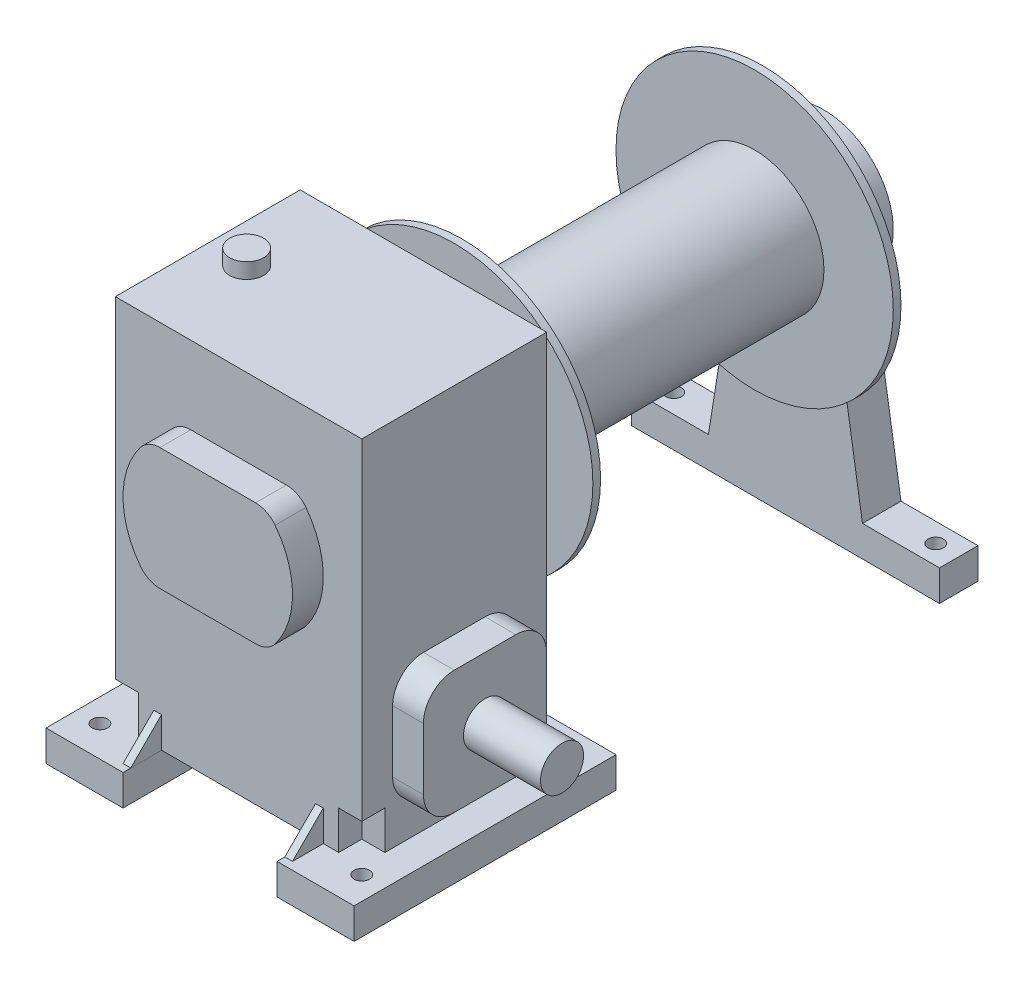
from build123d import *

# Parameters (mm, degrees)
EXTRUDE_1_DEPTH      = 20
EXTRUDE_1_DEPTH_BACK = 240
SKETCH_2_R           = 10
SKETCH_3_W           = 160
SKETCH_3_H           = 240
EXTRUDE_2_DEPTH      = 120
SKETCH_4_R           = 10
EXTRUDE_3_DEPTH      = 25
EXTRUDE_4_DEPTH      = 20
EXTRUDE_5_DEPTH      = 20
EXTRUDE_5_DEPTH_BACK = 180
SKETCH_7_W           = 80
SKETCH_7_H           = 80
FILLET_1_R           = 20
FILLET_2_R           = 16
SKETCH_8_R           = 14
EXTRUDE_6_DEPTH      = 50
SKETCH_10_W          = 50
SKETCH_10_H          = 20
EXTRUDE_7_DEPTH      = 85
EXTRUDE_7_2_DEPTH    = 85
EXTRUDE_8_DEPTH      = 5
SKETCH_12_R          = 5
CUT_EXTRUDE_1_DEPTH  = 20
SKETCH_13_W          = 15
SKETCH_13_H          = 15
CUT_EXTRUDE_2_DEPTH  = 25
SKETCH_14_R          = 11
EXTRUDE_9_DEPTH      = 10


with BuildPart() as part:
    # 草图1 → 旋转1 (revolve)
    with BuildSketch(Plane(origin=(0, 0, 0), x_dir=(0, 0, -1), z_dir=(1, 0, 0)), mode=Mode.PRIVATE) as revolve_1_sk:
        Polygon((-92.42282507, 0), (105.622076707, 0), (105.622076707, 90), (100.622076707, 90), (100.622076707, 45), (-89.377923293, 45), (-89.377923293, 90), (-94.377923293, 90), (-94.377923293, 0), align=None)
    revolve(revolve_1_sk.sketch.rotate(Axis((0, 0, 1000), (0, 0, -1)), 90), axis=Axis((0, 0, 1000), (0, 0, -1)))

    # 草图2 → 凸台-拉伸1 (add, two sides: drawn at the far end of the back side and taken through both)
    with BuildSketch(Plane.XY.offset(94.377923293).offset(-EXTRUDE_1_DEPTH_BACK)):
        Circle(SKETCH_2_R)
    extrude(amount=EXTRUDE_1_DEPTH + EXTRUDE_1_DEPTH_BACK)

    # 草图3 → 凸台-拉伸2 (add)
    with BuildSketch(Plane.XY.offset(114.377923293)):
        with Locations((0, -30)):
            Rectangle(SKETCH_3_W, SKETCH_3_H)
    extrude(amount=EXTRUDE_2_DEPTH)

    # 草图6 → 凸台-拉伸4 (add)
    with BuildSketch(Plane.XY.offset(234.377923293)):
        with BuildLine():
            Line((-38.147465423, 39.620334196), (38.147465423, 39.620334196))
            ThreePointArc((38.147465423, 39.620334196), (55, 0), (38.147465423, -39.620334196))
            Line((38.147465423, -39.620334196), (-38.147465423, -39.620334196))
            ThreePointArc((-38.147465423, -39.620334196), (-55, 0), (-38.147465423, 39.620334196))
        make_face()
    extrude(amount=EXTRUDE_4_DEPTH)

    # 草图7 → 凸台-拉伸5 (add, two sides: drawn at the far end of the back side and taken through both)
    with BuildSketch(Plane(origin=(80, 0, 0), x_dir=(0, 0, -1), z_dir=(1, 0, 0)).offset(-EXTRUDE_5_DEPTH_BACK)):
        with Locations((-174.377923293, -90)):
            Rectangle(SKETCH_7_W, SKETCH_7_H)
    extrude(amount=EXTRUDE_5_DEPTH + EXTRUDE_5_DEPTH_BACK)

    # 圆角1
    fillet_1_edges = [part.edges().sort_by_distance(p)[0] for p in [
        (90, -50, 134.377923293),
        (-90, -50, 134.377923293),
        (90, -130, 134.377923293),
        (-90, -130, 134.377923293),
        (90, -130, 214.377923293),
        (-90, -130, 214.377923293),
        (90, -50, 214.377923293),
        (-90, -50, 214.377923293),
    ]]
    fillet(fillet_1_edges, radius=FILLET_1_R)

    # 圆角2
    fillet_2_edges = [part.edges().sort_by_distance(p)[0] for p in [
        (-38.147465423, 39.620334196, 244.377923293),
        (-38.147465423, -39.620334196, 244.377923293),
        (38.147465423, -39.620334196, 244.377923293),
        (38.147465423, 39.620334196, 244.377923293),
    ]]
    fillet(fillet_2_edges, radius=FILLET_2_R)

    # 草图8 → 凸台-拉伸6 (add)
    with BuildSketch(Plane(origin=(100, 0, 0), x_dir=(0, 0, -1), z_dir=(1, 0, 0))):
        with Locations(Location((-174.377923293, -90, 0), (0, 0, 180))):
            Circle(SKETCH_8_R)
    extrude(amount=EXTRUDE_6_DEPTH)



with BuildPart() as body_2:
    # 草图4 → 凸台-拉伸3 (new body)
    with BuildSketch(Plane(origin=(0, 0, -145.622076707), x_dir=(-1, 0, 0), z_dir=(0, 0, -1))):
        with BuildLine():
            Line((-50, -150), (-100, -150))
            Line((-100, -150), (-100, -170))
            Line((-100, -170), (100, -170))
            Line((100, -170), (100, -150))
            Line((100, -150), (50, -150))
            Line((50, -150), (31.211895674, -32.416316392))
            ThreePointArc((31.211895674, -32.416316392), (41.40975311, -17.613413847), (45, 0))
            ThreePointArc((45, 0), (0, 45), (-45, 0))
            ThreePointArc((-45, 0), (-41.40975311, -17.613413847), (-31.211895674, -32.416316392))
            Line((-31.211895674, -32.416316392), (-50, -150))
        make_face()
        Circle(SKETCH_4_R, mode=Mode.SUBTRACT)
    extrude(amount=-EXTRUDE_3_DEPTH)


with BuildPart() as body_3:
    # 草图10 → 凸台-拉伸7 (new, symmetric)
    with BuildSketch(Plane.XY.offset(174.377923293)):
        with Locations((75, -160)):
            Rectangle(SKETCH_10_W, SKETCH_10_H)
    extrude(amount=EXTRUDE_7_DEPTH, both=True)


with BuildPart() as body_4:
    # 草图10 → Extrude 7 2 (new, symmetric)
    with BuildSketch(Plane.XY.offset(174.377923293)):
        with Locations((-75, -160)):
            Rectangle(SKETCH_10_W, SKETCH_10_H)
    extrude(amount=EXTRUDE_7_2_DEPTH, both=True)


with BuildPart() as part_1:
    add(part.part)

    add(body_3.part)  # 凸台-拉伸8 merges body 3
    # 草图11 → 凸台-拉伸8 (add)
    with BuildSketch(Plane.ZY.offset(-50)):
        Polygon((114.377923293, -130), (94.377923293, -150), (114.377923293, -150), align=None)
        Polygon((234.377923293, -130), (234.377923293, -150), (254.377923293, -150), align=None)
    extrude_8 = extrude(amount=-EXTRUDE_8_DEPTH)

    # 镜向1: 凸台-拉伸8 across plane
    add(extrude_8.mirror(Plane(origin=(0, 0, 0), x_dir=(0, 0, 1), z_dir=(1, 0, 0))))


with BuildPart() as cut_extrude_1_tool:
    # 草图12 → 切除-拉伸1 (new body)
    with BuildSketch(Plane.XZ.offset(170)):
        with Locations(Location((85, 239.377923293, 0), (0, 0, 270))):
            Circle(SKETCH_12_R)
        with Locations(Location((85, 109.377923293, 0), (0, 0, 270))):
            Circle(SKETCH_12_R)
        with Locations(Location((85, -133.122076707, 0), (0, 0, 270))):
            Circle(SKETCH_12_R)
        with Locations(Location((-85, -133.122076707, 0), (0, 0, 180))):
            Circle(SKETCH_12_R)
        with Locations(Location((-85, 109.377923293, 0), (0, 0, 270))):
            Circle(SKETCH_12_R)
        with Locations(Location((-85, 239.377923293, 0), (0, 0, 270))):
            Circle(SKETCH_12_R)
    extrude(amount=-CUT_EXTRUDE_1_DEPTH)


with BuildPart() as part_2:
    add(part_1.part)

    # 切除-拉伸1: cut by cut_extrude_1_tool
    add(cut_extrude_1_tool.part, mode=Mode.SUBTRACT)

    # 草图13 → 切除-拉伸2 (cut)
    with BuildSketch(Plane.XZ.offset(150)):
        with Locations((-72.5, 226.877923293)):
            Rectangle(SKETCH_13_W, SKETCH_13_H)
        with Locations((72.5, 226.877923293)):
            Rectangle(SKETCH_13_W, SKETCH_13_H)
        with Locations((72.5, 121.877923293)):
            Rectangle(SKETCH_13_W, SKETCH_13_H)
        with Locations((-72.5, 121.877923293)):
            Rectangle(SKETCH_13_W, SKETCH_13_H)
    extrude(amount=-CUT_EXTRUDE_2_DEPTH, mode=Mode.SUBTRACT)

    # 草图14 → 凸台-拉伸9 (add)
    with BuildSketch(Plane(origin=(0, 90, 0), x_dir=(1, 0, 0), z_dir=(0, 1, 0))):
        with Locations(Location((-54.750350248, -174.377923293, 0), (0, 0, 90))):
            Circle(SKETCH_14_R)
    extrude(amount=EXTRUDE_9_DEPTH)


with BuildPart() as body_2_1:
    add(body_2.part)

    # 切除-拉伸1: cut by cut_extrude_1_tool
    add(cut_extrude_1_tool.part, mode=Mode.SUBTRACT)


with BuildPart() as body_4_1:
    add(body_4.part)

    # 切除-拉伸1: cut by cut_extrude_1_tool
    add(cut_extrude_1_tool.part, mode=Mode.SUBTRACT)


solid = Compound([part_2.part, body_2_1.part, body_4_1.part])
